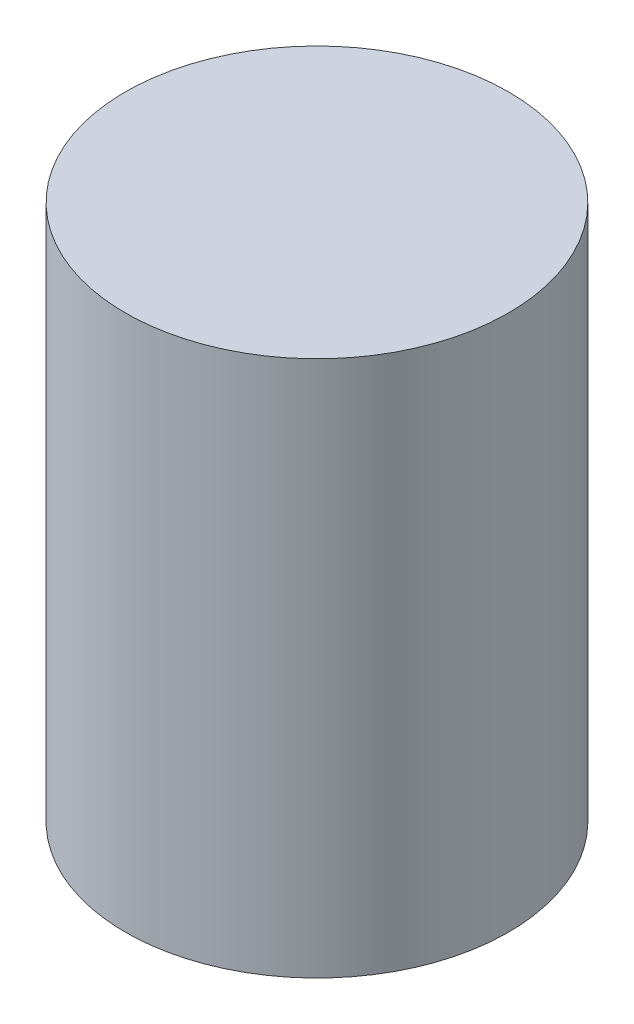
from build123d import *

# Parameters (mm, degrees)
SKETCH_1_W = 12.5
SKETCH_1_H = 35


with BuildPart() as part:
    # 草图1 → 旋转1 (revolve)
    with BuildSketch(Plane.XY, mode=Mode.PRIVATE) as revolve_1_sk:
        with Locations((-6.25, 17.5)):
            Rectangle(SKETCH_1_W, SKETCH_1_H)
    revolve(revolve_1_sk.sketch.rotate(Axis((0, 0, 0), (0, 1, 0)), 270), axis=Axis((0, 0, 0), (0, 1, 0)))


solid = part.part
